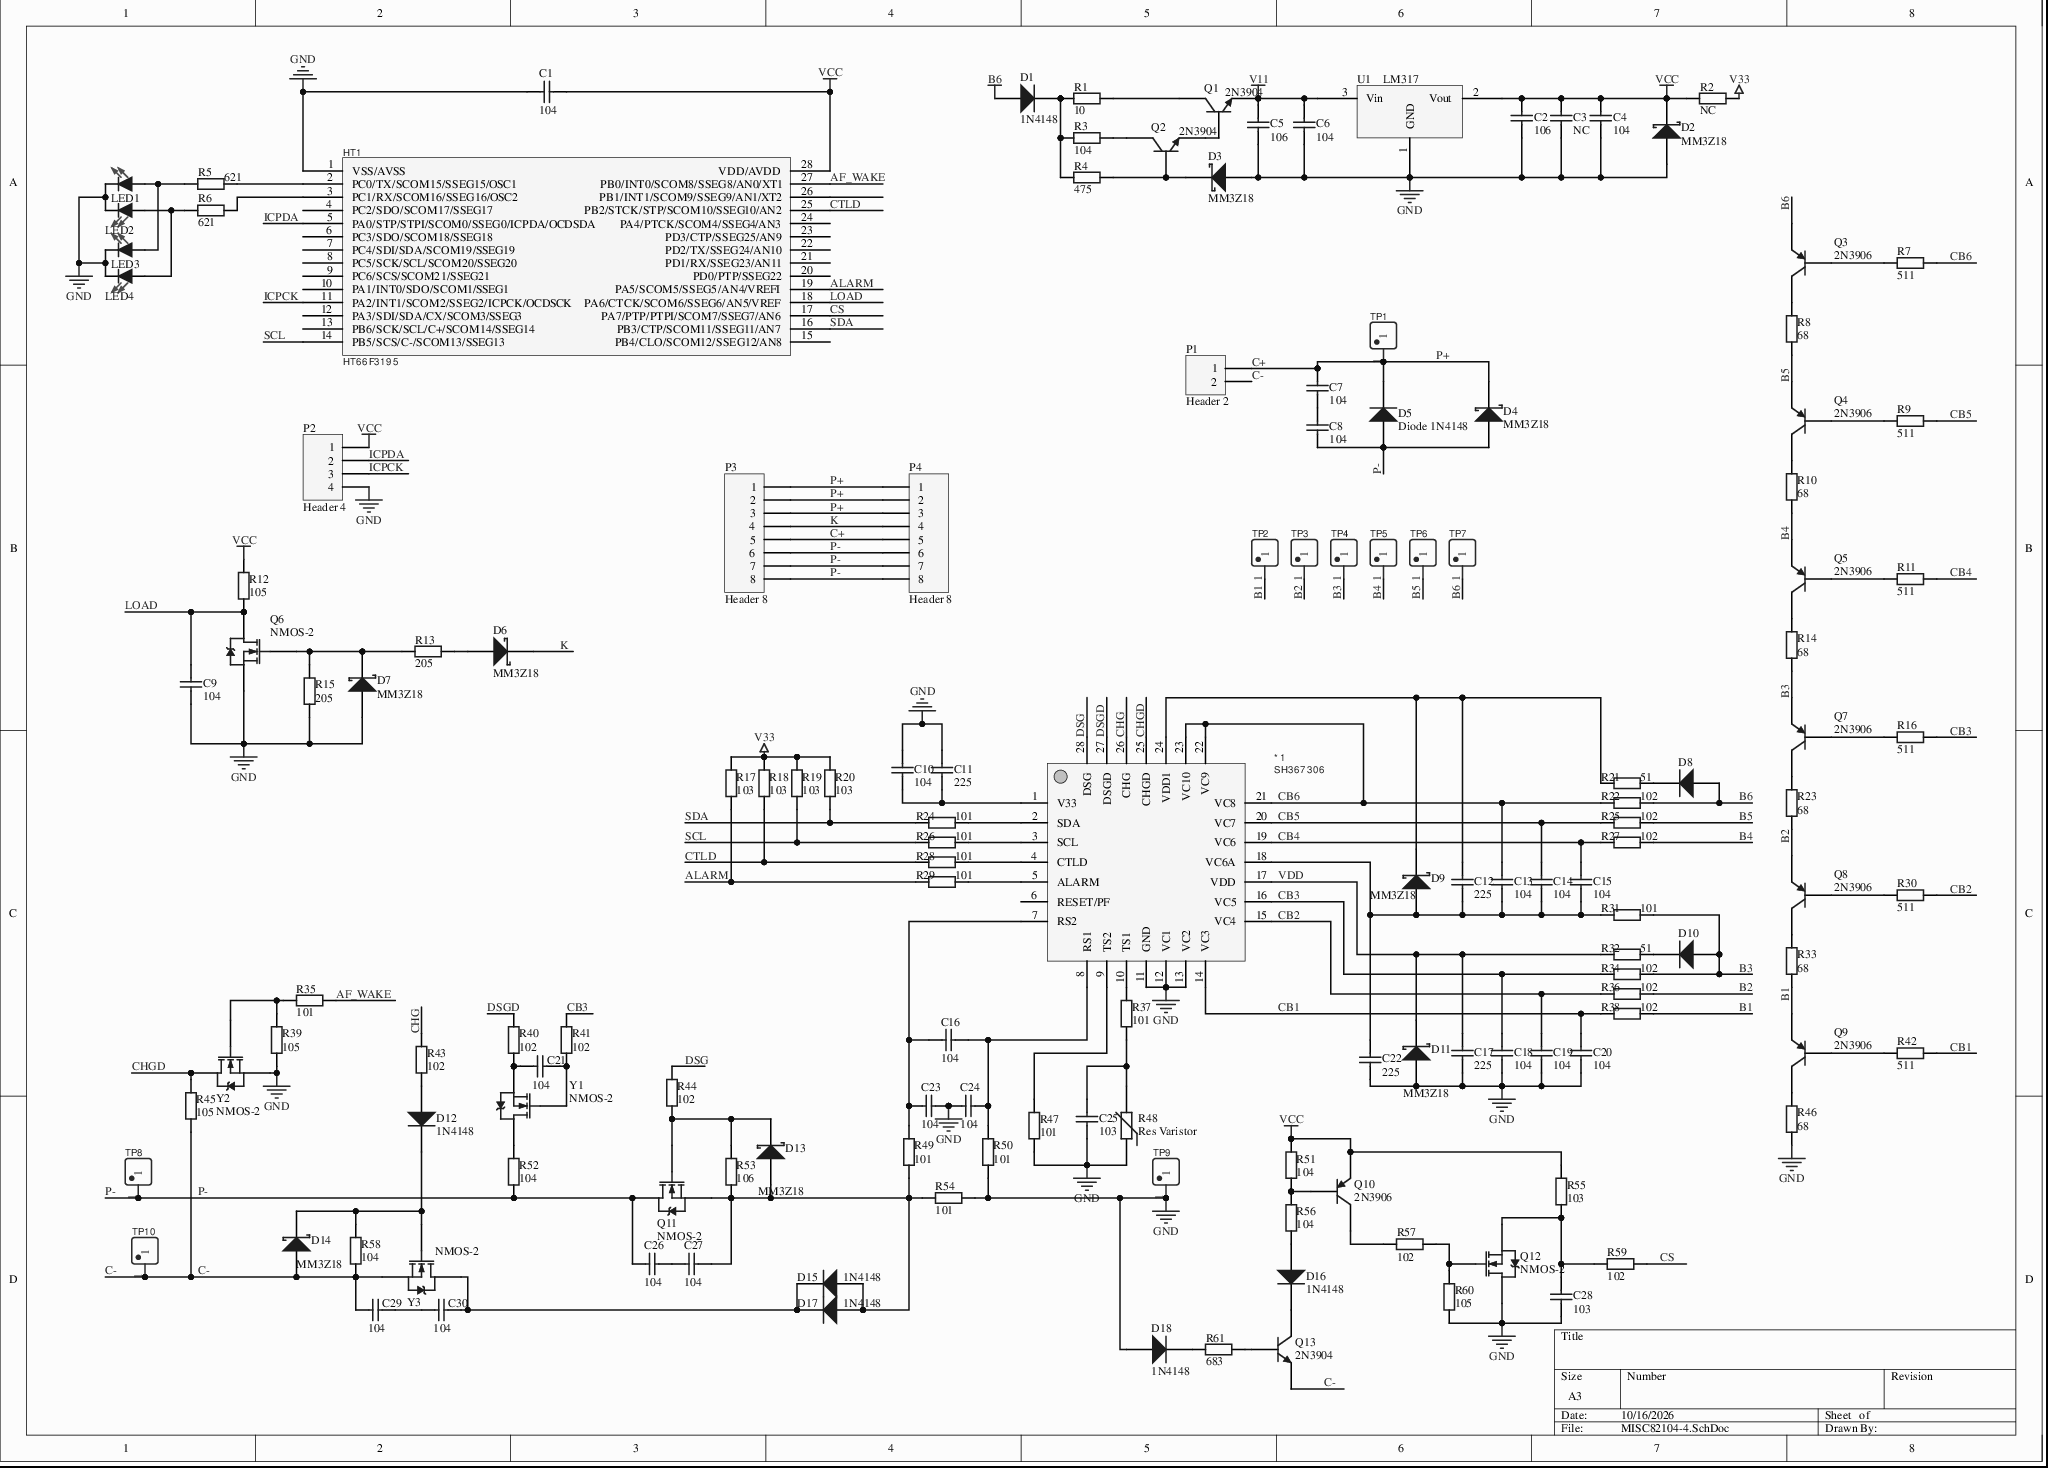
[diagram p0: MISC82104-4.SchDoc]
# Altium project MISC82104-8.PrjPcb
1 sheet, 146 parts. Net scope: global (net labels, ports and power ports of the same name join across sheets).
Board file: MISC82104.PcbDoc

## Sheet MISC82104-4.SchDoc
size A3

### Parts
*1  SH367306  [QFN28L(5*5)]
C1  104  [C0603]
C2  106  [C0603]
C3  NC  [C0603]
C4  104  [C0603]
C5  106  [C0603]
C6  104  [C0603]
C7  104  [C0603]
C8  104  [C0603]
C9  104  [C0603]
C10  104  [C0603]
C11  225  [C0603]
C12  225  [C0603]
C13  104  [C0603]
C14  104  [C0603]
C15  104  [C0603]
C16  104  [C0603]
C17  225  [C0603]
C18  104  [C0603]
C19  104  [C0603]
C20  104  [C0603]
C21  104  [C0603]
C22  225  [C0603]
C23  104  [C0603]
C24  104  [C0603]
C25  103  [C0603]
C26  104  [C0603]
C27  104  [C0603]
C28  103  [C0603]
C29  104  [C0603]
C30  104  [C0603]
D1  1N4148  [DO-35]
D2  MM3Z18  [TO-220AC]
D3  MM3Z18  [TO-220AC]
D4  MM3Z18  [TO-220AC]
D5  Diode 1N4148  [DO-35]
D6  MM3Z18  [TO-220AC]
D7  MM3Z18  [TO-220AC]
D8  Diode 1N4148  [DO-35]  (value not drawn)
D9  MM3Z18  [TO-220AC]
D10  Diode 1N4148  [DO-35]  (value not drawn)
D11  MM3Z18  [TO-220AC]
D12  1N4148  [DO-35]
D13  MM3Z18  [TO-220AC]
D14  MM3Z18  [TO-220AC]
D15  1N4148  [DO-35]
D16  1N4148  [DO-35]
D17  1N4148  [DO-35]
D18  1N4148  [DO-35]
HT1  HT66F3195  [SSOP28 - DUPLICATE]
LED1  I-LED  [I-LED-5MM]  (value not drawn)
LED2  I-LED  [I-LED-5MM]  (value not drawn)
LED3  I-LED  [I-LED-5MM]  (value not drawn)
LED4  I-LED  [I-LED-5MM]  (value not drawn)
P1  Header 2  [HDR1X2]
P2  Header 4  [HDR1X4]
P3  Header 8  [HDR1X8]
P4  Header 8  [HDR1X8]
Q1  2N3904  [TO-92A]
Q2  2N3904  [TO-92A]
Q3  2N3906  [TO-92A]
Q4  2N3906  [TO-92A]
Q5  2N3906  [TO-92A]
Q6  NMOS-2  [TO-220AB]
Q7  2N3906  [TO-92A]
Q8  2N3906  [TO-92A]
Q9  2N3906  [TO-92A]
Q10  2N3906  [TO-92A]
Q11  NMOS-2  [TO-220AB]
Q12  NMOS-2  [TO-220AB]
Q13  2N3904  [TO-92A]
R1  10  [AXIAL-0.4]
R2  NC  [AXIAL-0.4]
R3  104  [AXIAL-0.4]
R4  475  [AXIAL-0.4]
R5  621  [AXIAL-0.4]
R6  621  [AXIAL-0.4]
R7  511  [AXIAL-0.4]
R8  68  [AXIAL-0.4]
R9  511  [AXIAL-0.4]
R10  68  [AXIAL-0.4]
R11  511  [AXIAL-0.4]
R12  105  [AXIAL-0.4]
R13  205  [AXIAL-0.4]
R14  68  [AXIAL-0.4]
R15  205  [AXIAL-0.4]
R16  511  [AXIAL-0.4]
R17  103  [AXIAL-0.4]
R18  103  [AXIAL-0.4]
R19  103  [AXIAL-0.4]
R20  103  [AXIAL-0.4]
R21  51  [AXIAL-0.4]
R22  102  [AXIAL-0.4]
R23  68  [AXIAL-0.4]
R24  101  [AXIAL-0.4]
R25  102  [AXIAL-0.4]
R26  101  [AXIAL-0.4]
R27  102  [AXIAL-0.4]
R28  101  [AXIAL-0.4]
R29  101  [AXIAL-0.4]
R30  511  [AXIAL-0.4]
R31  101  [AXIAL-0.4]
R32  51  [AXIAL-0.4]
R33  68  [AXIAL-0.4]
R34  102  [AXIAL-0.4]
R35  101  [AXIAL-0.4]
R36  102  [AXIAL-0.4]
R37  101  [AXIAL-0.4]
R38  102  [AXIAL-0.4]
R39  105  [AXIAL-0.4]
R40  102  [AXIAL-0.4]
R41  102  [AXIAL-0.4]
R42  511  [AXIAL-0.4]
R43  102  [AXIAL-0.4]
R44  102  [AXIAL-0.4]
R45  105  [AXIAL-0.4]
R46  68  [AXIAL-0.4]
R47  101  [AXIAL-0.4]
R48  Res Varistor  [6-0805_N]
R49  101  [AXIAL-0.4]
R50  101  [AXIAL-0.4]
R51  104  [AXIAL-0.4]
R52  104  [AXIAL-0.4]
R53  106  [AXIAL-0.4]
R54  101  [AXIAL-0.4]
R55  103  [AXIAL-0.4]
R56  104  [AXIAL-0.4]
R57  102  [AXIAL-0.4]
R58  104  [AXIAL-0.4]
R59  102  [AXIAL-0.4]
R60  105  [AXIAL-0.4]
R61  683  [AXIAL-0.4]
TP1  TP-RED  [TEST-TH_BD2.54-P1.4_RED]  (value not drawn)
TP2  TP-RED  [TEST-TH_BD2.54-P1.4_RED]  (value not drawn)
TP3  TP-RED  [TEST-TH_BD2.54-P1.4_RED]  (value not drawn)
TP4  TP-RED  [TEST-TH_BD2.54-P1.4_RED]  (value not drawn)
TP5  TP-RED  [TEST-TH_BD2.54-P1.4_RED]  (value not drawn)
TP6  TP-RED  [TEST-TH_BD2.54-P1.4_RED]  (value not drawn)
TP7  TP-RED  [TEST-TH_BD2.54-P1.4_RED]  (value not drawn)
TP8  TP-RED  [TEST-TH_BD2.54-P1.4_RED]  (value not drawn)
TP9  TP-RED  [TEST-TH_BD2.54-P1.4_RED]  (value not drawn)
TP10  TP-RED  [TEST-TH_BD2.54-P1.4_RED]  (value not drawn)
U1  LM317  [TO220A]
Y1  NMOS-2  [TO-220AB]
Y2  NMOS-2  [TO-220AB]
Y3  NMOS-2  [TO-220AB]

### Nets
B6: D1.1(A) D8.1(A) Q3.1(E) R22.2 TP7.1
GND: *1.11(GND) *1.12(VC1) *1.13(VC2) C1.1 C2.1 C3.1 C4.1 C5.1 C6.1 C9.1 C10.2 C11.2 C17.1 C18.1 C19.1 C20.1 C22.1 C23.1 C24.2 C25.1 C28.2 D2.3(A) D3.3(A) D7.3(A) D11.3(A) D18.1(A) HT1.1(VSS/AVSS) LED1.2(K) LED2.2(K) LED3.2(K) LED4.2(K) P2.4 Q6.3(S) Q12.2(D) R15.1 R39.1 R46.2 R47.1 R48.1 R50.1 R54.1 R60.2 TP9.1 U1.1(GND) Y2.3(S)
V11: C5.2 C6.2 Q1.1(E) U1.3(Vin)
V33: R2.2 R17.2 R18.2 R19.2 R20.2
VCC: C1.2 C2.2 C3.2 C4.2 D2.1(K) HT1.28(VDD/AVDD) P2.1 Q10.1(E) R2.1 R12.2 R51.2 R55.1 U1.2(Vout)
AF_WAKE: HT1.27(PB0/INT0/SCOM8/SSEG8/AN0/XT1) R35.1
ALARM: HT1.19(PA5/SCOM5/SSEG5/AN4/VREFI) R17.1 R29.1
B1: Q9.1(E) R33.2 R38.2 TP2.1
B2: Q8.1(E) R23.2 R36.2 TP3.1
B3: D10.1(A) Q7.1(E) R14.2 R31.2 R34.2 TP4.1
B4: Q5.1(E) R10.2 R27.2 TP5.1
B5: Q4.1(E) R8.2 R25.2 TP6.1
C+: C7.2 D4.1(K) D5.2(K) P1.1 P3.1 P3.2 P3.3 P3.5 P4.1 P4.2 P4.3 P4.5 TP1.1  [also labelled P+]
C-: C29.2 D14.3(A) P1.2 Q13.1(E) R45.1 R58.1 TP10.1 Y3.3(S)
CB1: *1.14(VC3) C20.2 R38.1 R42.1
CB2: *1.15(VC4) C19.2 R30.1 R36.1
CB3: *1.16(VC5) C18.2 R16.1 R34.1 R41.2
CB4: *1.19(VC6) C15.2 R11.1 R27.1
CB5: *1.20(VC7) C14.2 R9.1 R25.1
CB6: *1.21(VC8) *1.22(VC9) *1.23(VC10) C13.2 R7.1 R22.1
CHG: *1.26(CHG) R43.2
CHGD: *1.25(CHGD) R45.2 Y2.2(D)
CS: HT1.17(PA7/PTP/PTPI/SCOM7/SSEG7/AN6) R59.2
CTLD: HT1.25(PB2/STCK/STP/SCOM10/SSEG10/AN2) R18.1 R28.1
DSG: *1.28(DSG) R44.2
DSGD: *1.27(DSGD) R40.2
ICPCK: HT1.11(PA2/INT1/SCOM2/SSEG2/ICPCK/OCDSCK) P2.3
ICPDA: HT1.5(PA0/STP/STPI/SCOM0/SSEG0/ICPDA/OCDSDA) P2.2
K: D6.1(K) P3.4 P4.4
LOAD: C9.2 HT1.18(PA6/CTCK/SCOM6/SSEG6/AN5/VREF) Q6.2(D) R12.1
P-: C8.1 C26.2 D4.3(A) D5.1(A) P3.6 P3.7 P3.8 P4.6 P4.7 P4.8 Q11.2(D) R52.1 TP8.1
SCL: HT1.14(PB5/SCS/C-/SCOM13/SSEG13) R19.1 R26.1
SDA: HT1.16(PB3/CTP/SCOM11/SSEG11/AN7) R20.1 R24.1
VDD: *1.17(VDD) C17.2 D11.1(K) R32.1
Net*1_1: *1.1(V33) C10.1 C11.1
Net*1_2: *1.2(SDA) R24.2
Net*1_3: *1.3(SCL) R26.2
Net*1_4: *1.4(CTLD) R28.2
Net*1_5: *1.5(ALARM) R29.2
Net*1_7: *1.7(RS2) C16.2 C23.2 R49.2
Net*1_8: *1.8(RS1) C16.1 C24.1 R50.2
Net*1_9: *1.9(TS2) R47.2
Net*1_10: *1.10(TS1) R37.2
Net*1_18: *1.18(VC6A) C12.1 C13.1 C14.1 C15.1 C22.2 D9.3(A) R31.1
Net*1_24: *1.24(VDD1) C12.2 D9.1(K) R21.1
NetC7_1: C7.1 C8.2
NetC21_1: C21.1 R41.1 Y1.1(G)
NetC21_2: C21.2 R40.1 Y1.3(S)
NetC25_2: C25.2 R37.1 R48.2
NetC26_1: C26.1 C27.2
NetC27_1: C27.1 D13.3(A) D15.1(A) D17.1(A) Q11.3(S) R49.1 R53.1 R54.2
NetC28_1: C28.1 Q12.3(S) R55.2 R59.1
NetC29_1: C29.1 C30.2
NetC30_1: C30.1 D15.2(K) D17.2(K) Y3.2(D)
NetD1_2: D1.2(K) R1.1 R3.1 R4.1
NetD3_1: D3.1(K) Q2.2(B) R4.2
NetD6_3: D6.3(A) R13.1
NetD7_1: D7.1(K) Q6.1(G) R13.2 R15.2
NetD8_2: D8.2(K) R21.2
NetD10_2: D10.2(K) R32.2
NetD12_1: D12.1(A) R43.1
NetD12_2: D12.2(K) D14.1(K) R58.2 Y3.1(G)
NetD13_1: D13.1(K) Q11.1(G) R44.1 R53.2
NetD16_1: D16.1(A) R56.1
NetD16_2: D16.2(K) Q13.3(C)
NetD18_2: D18.2(K) R61.2
NetHT1_2: HT1.2(PC0/TX/SCOM15/SSEG15/OSC1) R5.2
NetHT1_3: HT1.3(PC1/RX/SCOM16/SSEG16/OSC2) R6.2
NetLED1_1: LED1.1(A) LED3.1(A) R5.1
NetLED2_1: LED2.1(A) LED4.1(A) R6.1
NetQ1_2: Q1.2(B) Q2.1(E)
NetQ1_3: Q1.3(C) R1.2
NetQ2_3: Q2.3(C) R3.2
NetQ3_2: Q3.2(B) R7.2
NetQ3_3: Q3.3(C) R8.1
NetQ4_2: Q4.2(B) R9.2
NetQ4_3: Q4.3(C) R10.1
NetQ5_2: Q5.2(B) R11.2
NetQ5_3: Q5.3(C) R14.1
NetQ7_2: Q7.2(B) R16.2
NetQ7_3: Q7.3(C) R23.1
NetQ8_2: Q8.2(B) R30.2
NetQ8_3: Q8.3(C) R33.1
NetQ9_2: Q9.2(B) R42.2
NetQ9_3: Q9.3(C) R46.1
NetQ10_2: Q10.2(B) R51.1 R56.2
NetQ10_3: Q10.3(C) R57.2
NetQ12_1: Q12.1(G) R57.1 R60.1
NetQ13_2: Q13.2(B) R61.1
NetR35_2: R35.2 R39.2 Y2.1(G)
NetR52_2: R52.2 Y1.2(D)

Not connected (* = marked no-connect by the designer): *1 6(RESET/PF); HT1 4(PC2/SDO/SCOM17/SSEG17) 6(PC3/SDO/SCOM18/SSEG18) 7(PC4/SDI/SDA/SCOM19/SSEG19) 8(PC5/SCK/SCL/SCOM20/SSEG20) 9(PC6/SCS/SCOM21/SSEG21) 10(PA1/INT0/SDO/SCOM1/SSEG1) 12(PA3/SDI/SDA/CX/SCOM3/SSEG3) 13(PB6/SCK/SCL/C+/SCOM14/SSEG14) 15(PB4/CLO/SCOM12/SSEG12/AN8) 20(PD0/PTP/SSEG22) 21(PD1/RX/SSEG23/AN11) 22(PD2/TX/SSEG24/AN10) 23(PD3/CTP/SSEG25/AN9) 24(PA4/PTCK/SCOM4/SSEG4/AN3) 26(PB1/INT1/SCOM9/SSEG9/AN1/XT2)

### Library data of the parts
C1-C30 = Cap: Capacitor; Value: 100pF; Published: 8-Jun-2000; LatestRevisionDate: 17-Jul-2002; LatestRevisionNote: Re-released for DXP Platform.; PackageReference: RAD-0.3; PackageDescription: Radial Cap, Thru-Hole; 2 Leads; 0.3 in Pin Spacing; Publisher: Altium Limited
D1 D5 D8 D10 D12 D15-D18 = Diode 1N4148: High Conductance Fast Diode; Published: 8-Jun-2000; LatestRevisionDate: 17-Jul-2002; LatestRevisionNote: Re-released for DXP Platform.; DatasheetVersion: 1997; PackageReference: DO-35; PackageDescription: Diode, Axial; Body 3.8 x 1.9 mm (LxDia. max), Lead Dia. 0.53 mm (max); Code_JEDEC: DO-204-AH; ComponentLink1Description: Manufacturer Link; ComponentLink2Description: Datasheet; ComponentLink2URL: example.com/ds/1N%2F1N4148.pdf; Publisher: Altium Limited
D2-D4 D6 D7 D9 D11 D13 D14 = Diode 10TQ045: Schottky Rectifier; Note: Terminal 2 is the TAB and is electrically connected to the cathode; Published: 8-Jun-2000; LatestRevisionDate: 17-Jul-2002; LatestRevisionNote: Re-released for DXP Platform.; DatasheetVersion: PD-2.057B; PackageVersion: Feb-1998; PackageReference: TO-220AC; PackageDescription: TO, Thru-Hole, Vertical, Heatsink Mounted; 3 In-Line Leads (1 Absent); Pitch 2.54 mm; ComponentLink1Description: Manufacturer Link; ComponentLink2Description: Datasheet; ComponentLink2URL: example.com/product-info/datasheets/data/10tq.pdf; Publisher: Altium Limited
LED1-LED4 = I-LED: Infrared diode
P1 = Header 2: Header, 2-Pin; LatestRevisionDate: 17-Jul-2002; LatestRevisionNote: Re-released for DXP Platform.; Publisher: Altium Limited
P2 = Header 4: Header, 4-Pin; LatestRevisionDate: 17-Jul-2002; LatestRevisionNote: Re-released for DXP Platform.; Publisher: Altium Limited
P3 P4 = Header 8: Header, 8-Pin; LatestRevisionDate: 17-Jul-2002; LatestRevisionNote: Re-released for DXP Platform.; Publisher: Altium Limited
Q1 Q2 Q13 = 2N3904: NPN General Purpose Amplifier; Published: 8-Jun-2000; LatestRevisionDate: 15-Jan-2003; LatestRevisionNote: PCB Footprint 'BCY-W3/D4.7' replaced; DatasheetVersion: 1997; PackageVersion: Sep-1998; PackageReference: TO-92A; PackageDescription: TO, Flat Index; 3 In-Line, Axial Leads; Body Dia. 4.5mm; Leads 0.51 x 0.48 mm (max); ComponentLink1Description: Manufacturer Link; ComponentLink2Description: Datasheet; ComponentLink2URL: example.com/ds/2N%2F2N3904.pdf; Publisher: Altium Limited
Q3-Q5 Q7-Q10 = 2N3906: PNP General Purpose Amplifier; Published: 8-Jun-2000; LatestRevisionDate: 15-Jan-2003; LatestRevisionNote: PCB Footprint 'BCY-W3/D4.7' replaced; DatasheetVersion: 1997; PackageVersion: Sep-1998; PackageReference: TO-92A; PackageDescription: TO, Flat Index; 3 In-Line, Axial Leads; Body Dia. 4.5mm; Leads 0.51 x 0.48 mm (max); ComponentLink1Description: Manufacturer Link; ComponentLink2Description: Datasheet; ComponentLink2URL: example.com/ds/2N%2F2N3906.pdf; Publisher: Altium Limited
Q6 Q11 Q12 Y1-Y3 = NMOS-2: N-Channel Power MOSFET; Note: Pin 2 is electrically connected to pin 4.; Published: 8-Jun-2000; LatestRevisionDate: 17-Jul-2002; LatestRevisionNote: Re-released for DXP Platform.; DatasheetVersion: PD-9.814; PackageVersion: Feb-1997; PackageReference: TO-220AB; PackageDescription: TO, Thru-Hole, Vertical, Heatsink Mounted; 3 In-Line Leads; Pitch 2.54 mm; ComponentLink1Description: Manufacturer Link; Publisher: Altium Limited
R1-R47 R49-R61 = Res2: Resistor; Value: 1K; Published: 8-Jun-2000; LatestRevisionDate: 17-Jul-2002; LatestRevisionNote: Re-released for DXP Platform.; PackageReference: AXIAL-0.4; PackageDescription: Axial Device, Thru-Hole; 2 Leads; 0.4 in Pin Spacing; Publisher: Altium Limited
R48 = Res Varistor: Varistor (Voltage-Sensitive Resistor); Published: 24-Mar-1999; LatestRevisionDate: 29-May-2009; LatestRevisionNote: IPC-7351 Footprint Added.; PackageVersion: Mar-2003; PackageReference: 6-0805; PackageDescription: Chip Resistor 0805 Case Size; Code_IPC: RESC2012; Publisher: Altium Limited
U1 = LM317: Adjustable linear voltage regulator IC